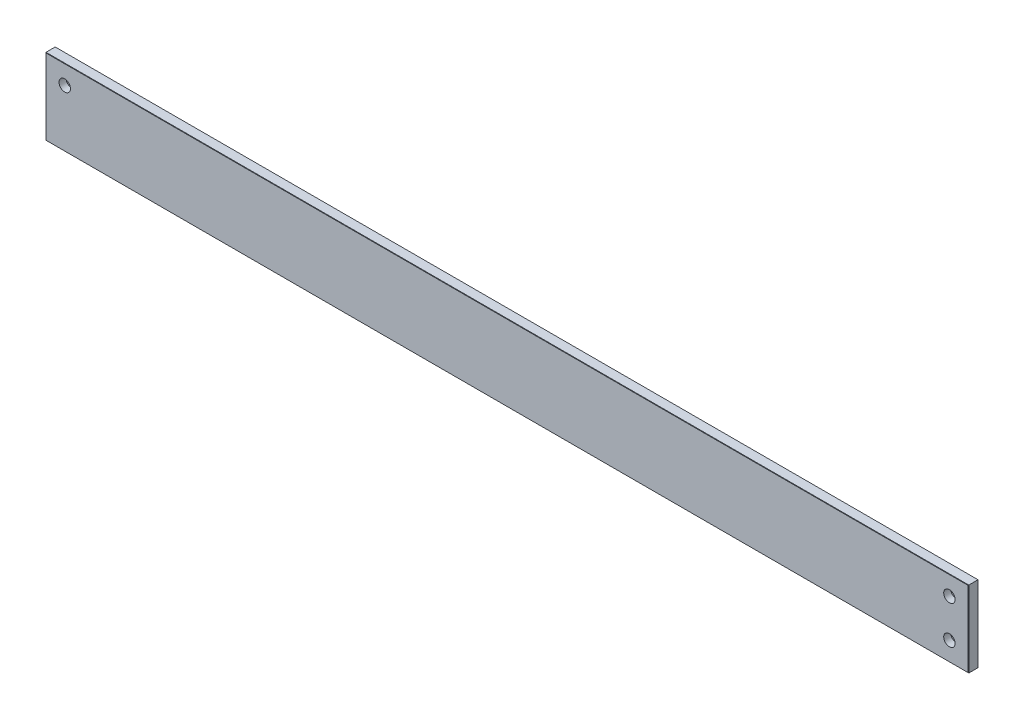
SolidWorks part; units mm, degrees
material "普通碳钢"
ref_plane "前视基准面" through (0, 0, 0) normal (0, 0, 1) x (1, 0, 0)
ref_plane "上视基准面" through (0, 0, 0) normal (0, 1, 0) x (1, 0, 0)
ref_plane "右视基准面" through (0, 0, 0) normal (1, 0, 0) x (0, 0, -1)
sketch "草图1" plane through (0, 0, 0) normal (0, 0, 1) x (1, 0, 0)
  line L1 (-726.5, 60) -> (726.5, 60)
  line L2 (-726.5, 60) -> (-726.5, -60)
  line L3 (-726.5, -60) -> (726.5, -60)
  line L4 (726.5, 60) -> (726.5, -60)
  line L5 (-726.5, 60) -> (726.5, -60) construction
  line L6 (-726.5, -60) -> (726.5, 60) construction
  point P0 (0, 0)
  dimension "D1" = 1453
  dimension "D2" = 120
extrude "凸台-拉伸1" add sketch "草图1" along normal mid plane 15
hole_wizard "打孔尺寸(%根据)内六角圆柱头螺钉的类型1" positions "3D草图1" profile "草图2" counterbore size "M10" standard "GB" end condition through all
sketch3d "3D草图1"
  line L0 (726.5, 60, 7.5) -> (-726.5, 60, 7.5) construction
  line L1 (-726.5, 60, 7.5) -> (-726.5, -60, 7.5) construction
  point P0 (-696.5, 30, 7.5)
  dimension "D1" = 30
  dimension "D2" = 30
sketch "草图2" plane through (-696.5, 30, 7.5) normal (1, 0, 0) x (0, -1, 0)
  line L0 (0, 0) -> (0, 15)
  line L1 (0, 15) -> (5.5, 15)
  line L3 (5.5, 15) -> (5.5, 11)
  line L4 (5.5, 11) -> (9, 11)
  line L5 (9, 11) -> (9, 0)
  line L7 (9, 0) -> (0, 0)
  line L11 (0, -6.35) -> (0, 107.95) construction
  dimension "通孔孔直径" = 11
  dimension "通孔孔深度" = 15
  dimension "柱形沉头孔直径" = 18
  dimension "柱形沉头孔深度" = 11
hole_wizard "打孔尺寸(%根据)内六角圆柱头螺钉的类型2" positions "3D草图2" profile "草图3" counterbore size "M10" standard "GB" end condition through all
sketch3d "3D草图2"
  line L0 (726.5, -60, 7.5) -> (726.5, 60, 7.5) construction
  line L1 (726.5, 60, 7.5) -> (-726.5, 60, 7.5) construction
  line L2 (-726.5, -60, 7.5) -> (726.5, -60, 7.5) construction
  point P0 (696.5, 30, 7.5)
  point P2 (696.5, -30, 7.5)
  dimension "D1" = 30
  dimension "D2" = 30
  dimension "D3" = 30
  dimension "D4" = 30
sketch "草图3" plane through (696.5, 30, 7.5) normal (1, 0, 0) x (0, -1, 0)
  line L0 (0, 0) -> (0, 15)
  line L1 (0, 15) -> (5.5, 15)
  line L3 (5.5, 15) -> (5.5, 11)
  line L4 (5.5, 11) -> (9, 11)
  line L5 (9, 11) -> (9, 0)
  line L7 (9, 0) -> (0, 0)
  line L11 (0, -6.35) -> (0, 107.95) construction
  dimension "通孔孔直径" = 11
  dimension "通孔孔深度" = 15
  dimension "柱形沉头孔直径" = 18
  dimension "柱形沉头孔深度" = 11
chamfer "倒角1" distance 0.5 angle 45 4 edges at (726.5, 0, 7.5) (0, -60, 7.5) (-726.5, 0, 7.5) (0, 60, 7.5)
